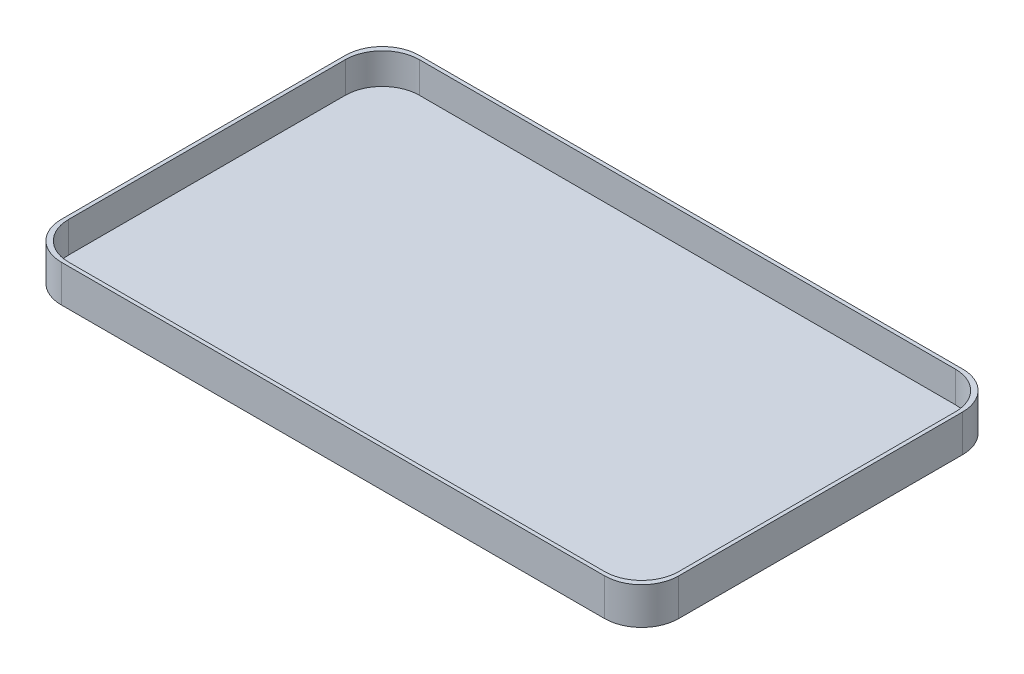
SolidWorks part; units mm, degrees
ref_plane "Front Plane" through (0, 0, 0) normal (0, 0, 1) x (1, 0, 0)
ref_plane "Top Plane" through (0, 0, 0) normal (0, 1, 0) x (1, 0, 0)
ref_plane "Right Plane" through (0, 0, 0) normal (1, 0, 0) x (0, 0, -1)
other "Configuration Table"
sketch "Sketch1" plane through (0, 0, 0) normal (0, 1, 0) x (1, 0, 0)
  line L1 (-220, 145) -> (220, 145)
  line L2 (-250, 115) -> (-250, -115)
  line L3 (-220, -145) -> (220, -145)
  line L4 (250, 115) -> (250, -115)
  line L5 (-250, 145) -> (250, -145) construction
  line L6 (-250, -145) -> (250, 145) construction
  arc A0 (250, 115) -> (220, 145) centre (220, 115) ccw
  arc A1 (220, -145) -> (250, -115) centre (220, -115) ccw
  arc A2 (-220, -145) -> (-250, -115) centre (-220, -115) cw
  arc A3 (-250, 115) -> (-220, 145) centre (-220, 115) cw
  point P0 (0, 0)
  dimension "D3" = 30
  dimension "D1" = 290
  dimension "D2" = 500
extrude "Boss-Extrude1" add sketch "Sketch1" along normal blind 30
sketch "Sketch2" plane through (0, 30, 0) normal (0, 1, 0) x (1, 0, 0)
  line L1 (-217, 142) -> (217, 142)
  line L2 (-247, 112) -> (-247, -112)
  line L3 (-217, -142) -> (217, -142)
  line L4 (247, 112) -> (247, -112)
  line L5 (-247, 142) -> (247, -142) construction
  line L6 (-247, -142) -> (247, 142) construction
  arc A0 (247, -112) -> (217, -142) centre (217, -112) cw
  arc A1 (217, 142) -> (247, 112) centre (217, 112) cw
  arc A2 (-217, -142) -> (-247, -112) centre (-217, -112) cw
  arc A3 (-217, 142) -> (-247, 112) centre (-217, 112) ccw
  point P0 (0, 0)
  dimension "D3" = 30
  dimension "D1" = 494
  dimension "D2" = 284
extrude "Cut-Extrude1" cut sketch "Sketch2" against normal blind 25
